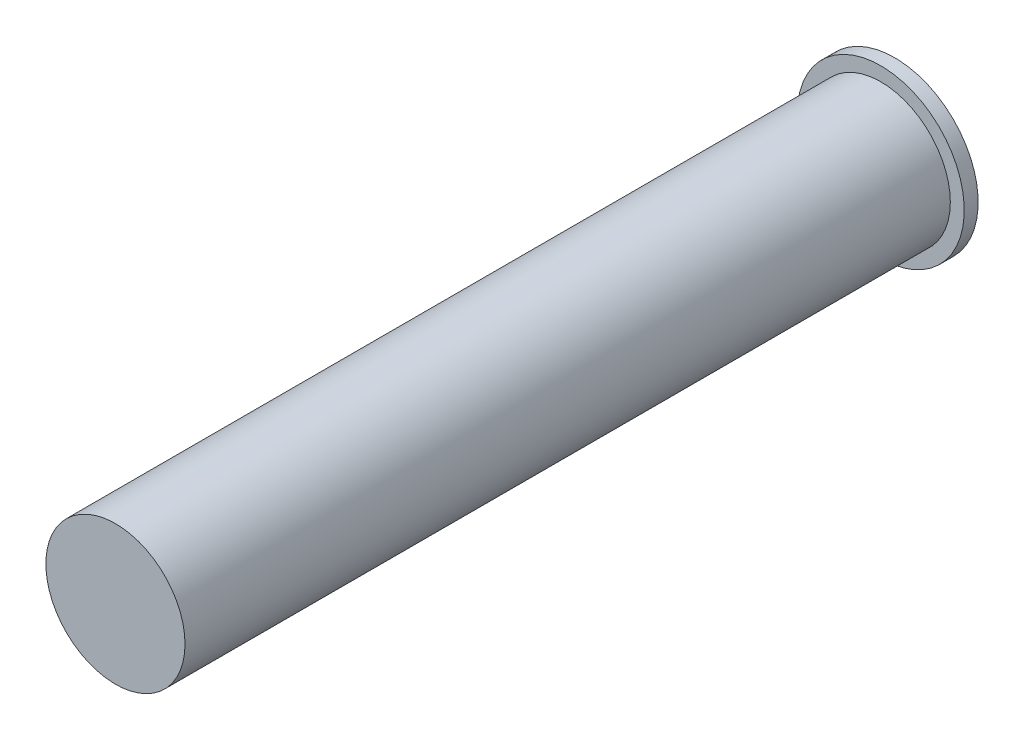
SolidWorks part; units mm, degrees
ref_plane "前视基准面" through (0, 0, 0) normal (0, 0, 1) x (1, 0, 0)
ref_plane "上视基准面" through (0, 0, 0) normal (0, 1, 0) x (1, 0, 0)
ref_plane "右视基准面" through (0, 0, 0) normal (1, 0, 0) x (0, 0, -1)
sketch "草图1" plane through (0, 0, 0) normal (0, 0, 1) x (1, 0, 0)
  circle A0 centre (0, 0) radius 5
  dimension "D1" = 10
extrude "凸台-拉伸1" add sketch "草图1" along normal blind 55
sketch "草图2" plane through (0, 0, 0) normal (0, 0, -1) x (-1, 0, 0)
  circle A0 centre (0, 0) radius 6
  dimension "D1" = 12
extrude "凸台-拉伸2" add sketch "草图2" along normal blind 1
